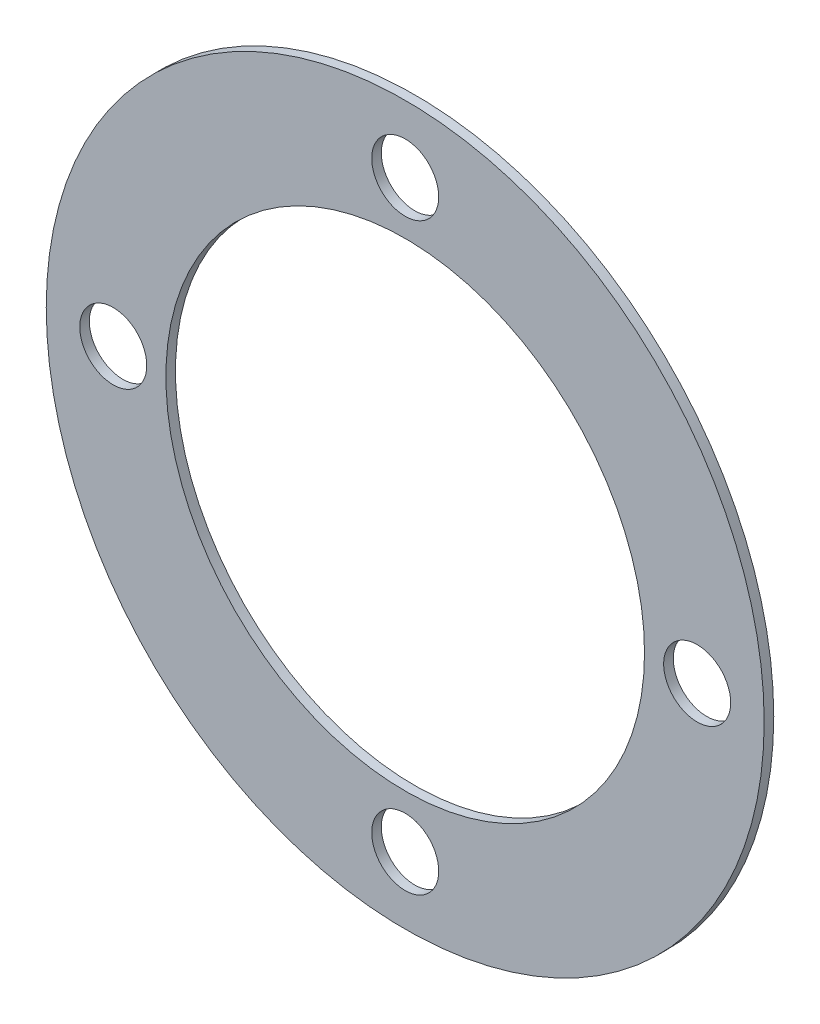
from build123d import *

# Parameters (mm, degrees)
SKETCH1_R           = 37.5
SKETCH1_R_2         = 25
SKETCH1_R_3         = 3.5
BOSS_EXTRUDE1_DEPTH = 1


with BuildPart() as part:
    # Sketch1 → Boss-Extrude1 (new body)
    with BuildSketch(Plane.XY):
        Circle(SKETCH1_R)
        Circle(SKETCH1_R_2, mode=Mode.SUBTRACT)
        with Locations((0, 30.5)):
            Circle(SKETCH1_R_3, mode=Mode.SUBTRACT)
        with Locations((30.5, 0)):
            Circle(SKETCH1_R_3, mode=Mode.SUBTRACT)
        with Locations((0, -30.5)):
            Circle(SKETCH1_R_3, mode=Mode.SUBTRACT)
        with Locations((-30.5, 0)):
            Circle(SKETCH1_R_3, mode=Mode.SUBTRACT)
    extrude(amount=BOSS_EXTRUDE1_DEPTH)


solid = part.part
